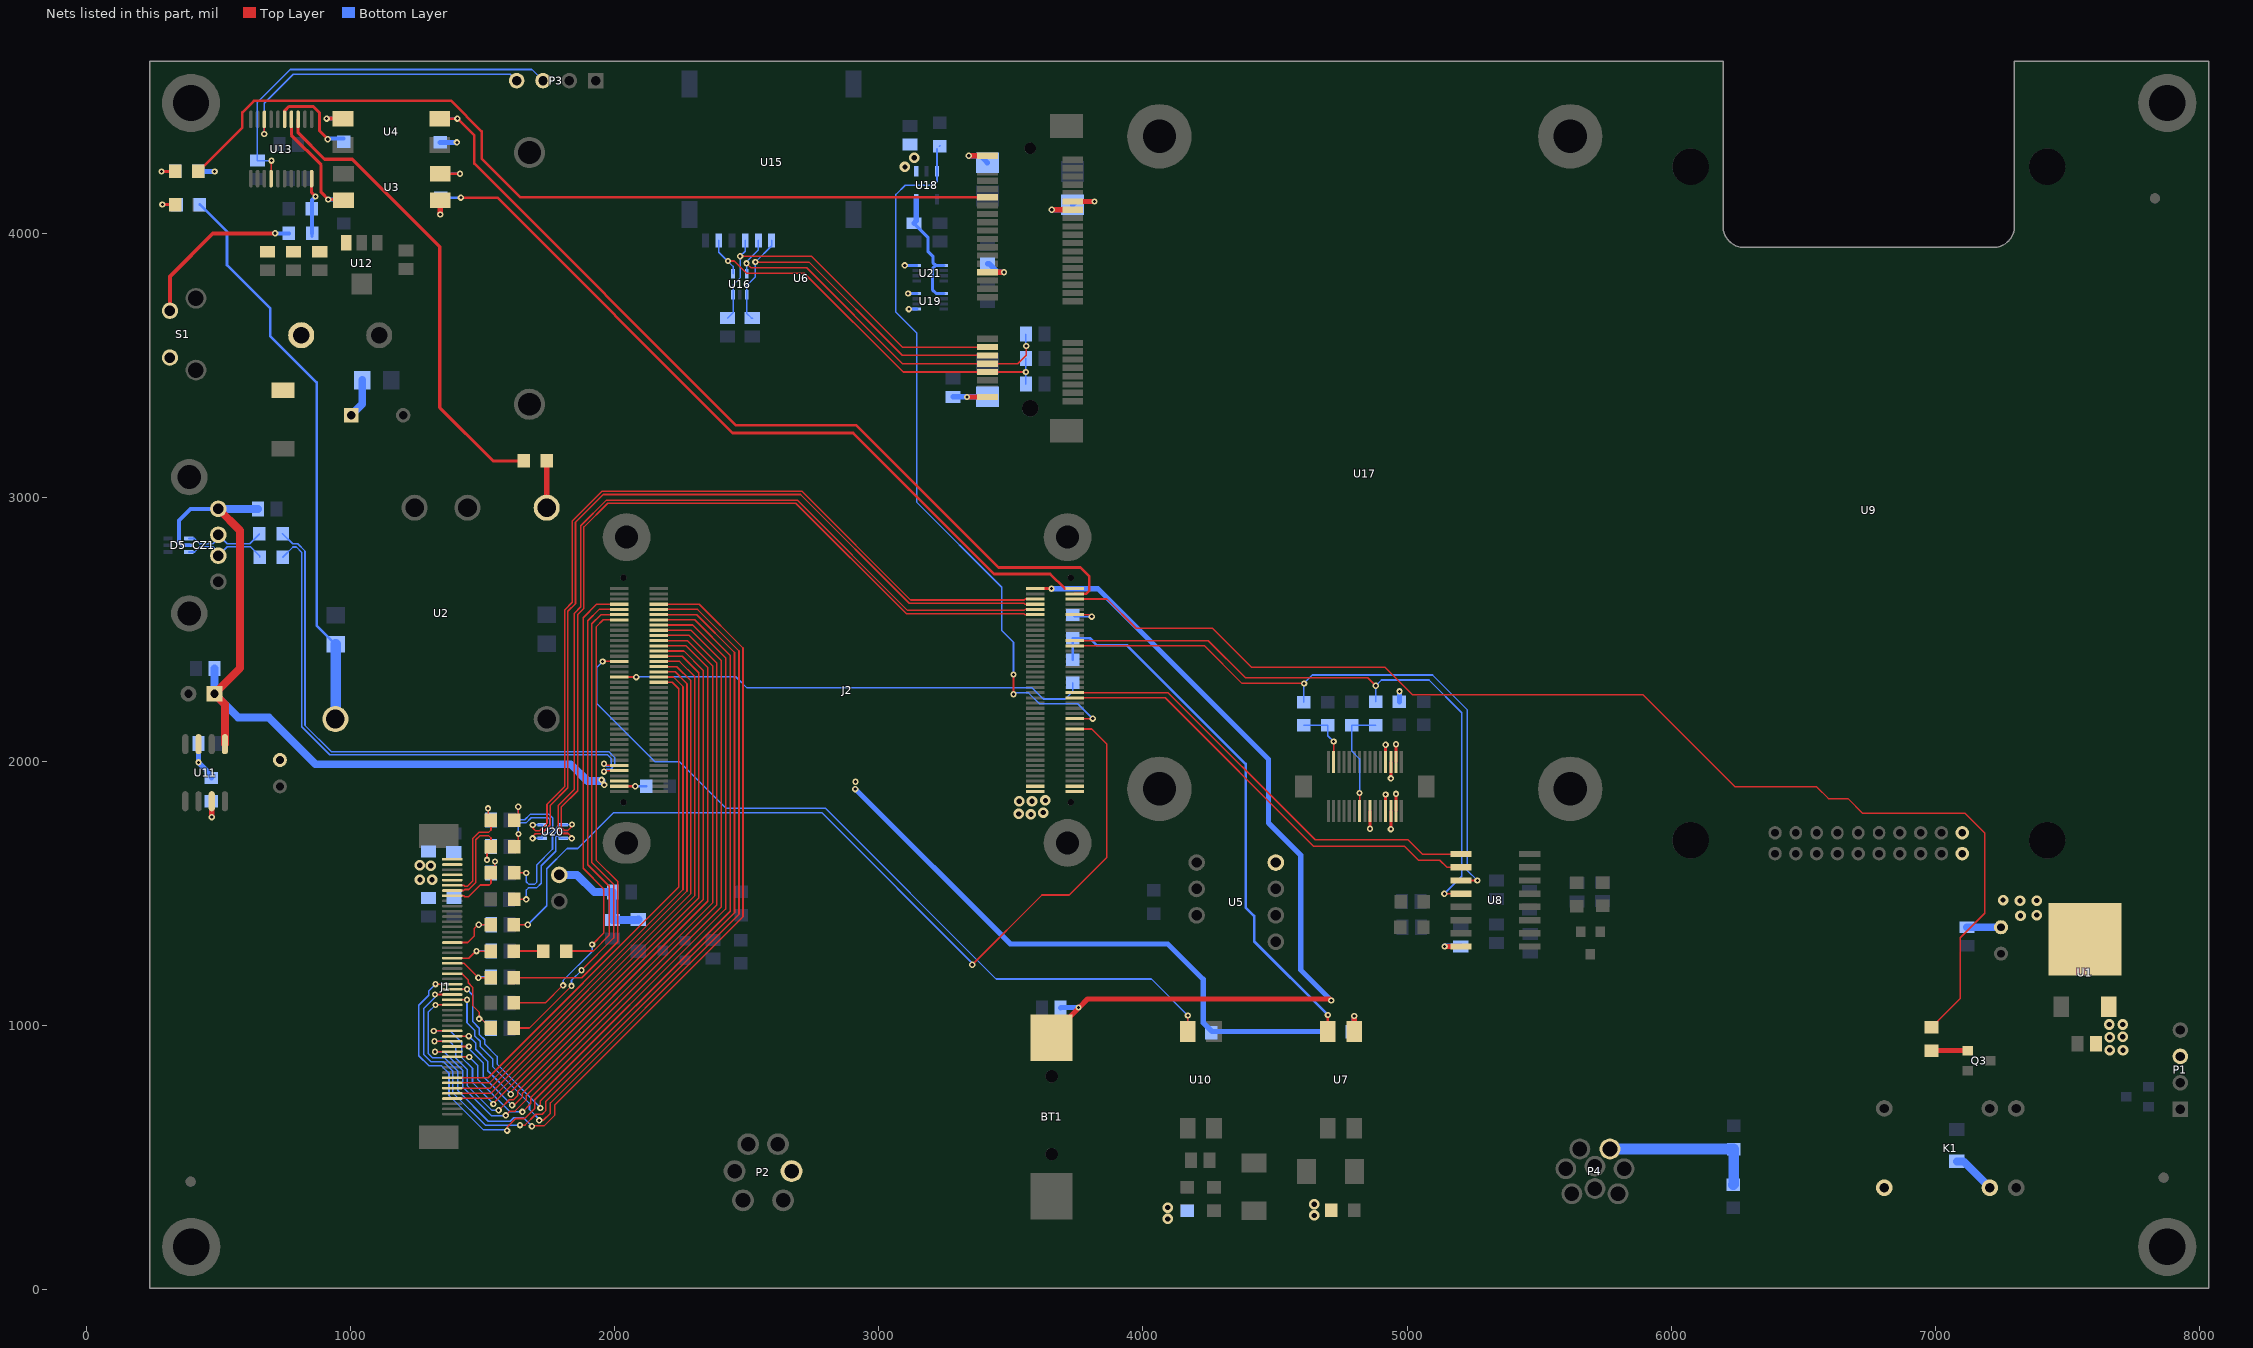
[diagram p0: the nets of this part, all layers, seen from the top]
# Altium PCB MISC82794.PcbDoc (part 4 of 5)
Units mil, origin at the board's own origin, x right, y up, seen from the top; angles counter-clockwise.
Board outline 7795.28 x 4645.67 mil, 4 copper layers (Top Layer, GND, POWER, Bottom Layer); 157 components, 133 nets, 768 pads, 456 vias.

## Via types
v1: diameter 24, hole 12, Top Layer to Bottom Layer, 258 vias
v2: diameter 40, hole 20, Top Layer to Bottom Layer, 197 vias
v3: diameter 30, hole 15, Top Layer to Bottom Layer, 1 vias

## Nets (pads, with @x,y where several pads share a name; then routed paths per layer and width w, separated by ;. In a path a pad name is that pad's centre, name@x,y a point inside that pad or via, vN(x,y) a via of type N, cw(c..) or ccw(c..) an arc to the next point about the centre after c; other vN are vias at no path point) (continued)
NetDD1_1: DD1.1 R1.1 | length 103
  Top Layer w10: v1(288.14,4108.86) DD1.1@337.14,4108.86
  Bottom Layer w10: v1(288.14,4108.86) R1.1@342.14,4108.86
NetDD2_1: DD2.1 R45.2 | length 102
  Top Layer w10: v1(285,4234) DD2.1@336,4234
  Bottom Layer w10: v1(285,4234) R45.2@336,4234
NetDD2_2: DD2.2 U6.42 | length 3342.4
  Top Layer w10: DD2.2@424,4234 591,4401 591,4457 635,4501 1382,4501 1497,4386 1497,4283 1643.79,4136.21 U6.42@3411.58,4136.21
NetJ2_A35: J2.A35 R37.2 | length 1796.2
  Top Layer w6: J2.A35@2017.8,2320.21 v1@2081.79,2320.21
  Bottom Layer w6: v1(2082,2320) 2083.53,2321.53 2459,2321.53 2501.53,2279 3581,2279 3623,2237 3671,2237 3706,2237 3734,2265 R37.2@3734,2298
NetJ2_B69: J2.B69 R36.2 | length 141.4
  Top Layer w6: J2.B69@3742.2,2556.43 3798.57,2556.43 v1(3806,2549)
  Bottom Layer w6: R36.2@3734,2555 3740,2549 v1(3806,2549)
NetL1_1: L1.1 R5.2 | length 110.2
  Top Layer w6: L1.1@1619,1282.6 1619.4,1283 R5.2@1729,1283
NetP4_3: P4.3 R39.1 R40.1 | length 601.8
  Bottom Layer w40: P4.3@5768.09,533.49 R40.1@6235.51,533.49 ; R39.1@6235,399 6236,400 R40.1@6236,533
NetQ3_1: Q3.1 R30.2 | length 122.7
  Top Layer w19.68: R30.2@7000,906 7121.9,906 Q3.1@7122.5,905.4
NetR8_1: R8.1 U2.6 | length 177
  Top Layer w6: R8.1@1744,3137 R8.1@1744,3138
  Top Layer w20: U2.6@1743,2961 R8.1@1743,3137
NetR8_2: R8.2 U13.13 | length 1776.4
  Top Layer w12: U13.13@801.98,4431.2 801.98,4380.02 902,4280 1006.92,4280 1338,3948.92 1338,3340 1540,3138 R8.2@1656,3138
NetR11_2: R11.2 U3.2 | length 148.8
  Top Layer w10: U3.2@1340.07,4225 v1(1415,4225)
  Bottom Layer w10: R11.2@1342,4223 1344,4225 v1(1415,4225)
NetR18_2: R18.2 U7.1 | length 122.1
  Top Layer w20: U7.1@4800,978.07 v1(4800,1037)
  Bottom Layer w20: R18.2@4790,978 4800,988 v1(4800,1037)
NetR24_1: R24.1 U11.3 | length 120.4
  Top Layer w20: v1(475,1790) U11.3@475,1849.97
  Bottom Layer w20: R24.1@474,1850 474,1791 v1(475,1790)
NetR29_1: R29.1 U4.1 | length 125.9
  Top Layer w15: v1(910,4434) U4.1@971.93,4434
  Bottom Layer w15: v1(910,4434) R29.1@974,4434
NetR29_2: R29.2 U13.15 | length 356.2
  Top Layer w12: U13.15@750.8,4431.2 750.8,4463.8 767,4480 859.77,4480 883,4456.77 883,4388 915,4356 v1(914,4356)
  Bottom Layer w15: v1@914,4358 R29.2@974,4358
NetR31_1: R31.1 S1.1 | length 699
  Top Layer w15: S1.1@316.79,3706.58 316.79,3836.79 480,4000 642,4000 ; 591,4000 642,4000 ; v1(715,4000) 642,4000
  Bottom Layer w15: v1(715,4000) R31.1@767,4000
NetR31_2: R31.2 R34.2 U13.10 | length 230.3
  Top Layer w12: U13.10@853.16,4206.79 853.16,4153.84 v1(868,4139)
  Bottom Layer w12: R31.2@854,3988 R31.2@854,4000
  Bottom Layer w15: R31.2@855,4000 855,4126 v1(868,4139)
NetR33_2: R33.2 U3.4 U13.14 | length 478.2
  Top Layer w12: U13.14@776.39,4431.2 776.39,4371.61 889,4259 889,4155 v1(916,4128) 970.93,4128 U3.4@973.93,4125
  Bottom Layer w15: v1(916,4128) R33.2@974,4128
NetR41_2: R41.2 R42.2 U17.3 | length 238.5
  Top Layer w6: U17.3@4721.89,1998.52 v1(4721.89,2075.89)
  Bottom Layer w6: R41.2@4609,2137 R42.2@4700,2137 4700,2097.78 v1(4721.89,2075.89)
NetR43_2: R43.2 R44.2 U17.14 | length 428.1
  Top Layer w6: v1(4820,1881) 4820.31,1880.69 U17.14@4820.31,1813.48
  Bottom Layer w6: v1(4820,1881) 4820,2010 4790,2040 R43.2@4790,2138 R44.2@4881,2138
OVER_LOAD: J2.A29 R21.2 U10.4 | length 3084.3
  Top Layer w6: v1(1954.73,2379.27) J2.A29@2017.8,2379.27 ; U10.4@4169,978.07 4170,979.07 v1(4170,1039)
  Bottom Layer w6: v1(1954.73,2379.27) 1933,2357.54 1933,2219.3 2152.3,2000 2245,2000 2421,1824 2797,1824 3444,1177 4032,1177 v1(4170,1039) R21.2@4170,974
POW_CTRL: J2.B75 R30.1 | length 4648.2
  Top Layer w6: J2.B75@3742.2,2615.49 3863.51,2615.49 3974.5,2504.5 4263.5,2504.5 4410,2358 4915,2358 5020,2253 5893,2253 6241,1905 6550,1905 6595,1860 6669,1860 6724,1805 7112,1805 7187,1730 7187,1426 7094,1333 7094,1103 R30.1@6985,994 ; R30.1@6983,977 R30.1@6983,994
POW_OFF: J2.B79 R11.1 | length 3019.3
  Top Layer w10: v1(1418,4135) 1433,4135 ; 1439,4135 1433,4135 ; J2.B79@3742.2,2654.86 3704.14,2654.86 3649,2710 3437,2710 2903,3244 2447,3244 1556,4135 1433,4135
  Bottom Layer w10: R11.1@1342,4135 v1(1418,4135)
POW_SW: J2.B77 R28.2 U4.4 | length 3418.3
  Top Layer w10: U4.4@1338.07,4434 v1(1405,4434) 1469,4370 1469,4264 2460,3273 2915,3273 3453,2735 3763,2735 3797,2701 3797,2647.17 3785,2635.17 J2.B77@3742.2,2635.17
  Bottom Layer w10: R28.2@1340,4432 1342,4434 v1(1405,4434)
POWER_OK: J2.B29 R46.1 U18.3 | length 2788.8
  Top Layer w6: v1(3510,2255) v1(3510,2330) ; J2.B29@3742.2,2162.73 v1(3809.73,2162.73)
  Bottom Layer w6: R46.1@3220.37,4320.37 U18.3@3220.37,4235.15 3220.37,4195.37 3207,4182 3100,4182 3065,4147 3065,3701 3143,3623 3143,2983 3466,2660 3466,2496 3510,2452 v1(3510,2330) ; R46.1@3230,4330 R46.1@3231.73,4331.73 ; v1(3510,2255) 3515,2260 3567,2260 3608,2219 3753.47,2219 v1(3809.73,2162.73)
PWM_LIGHT: C8.1 J1.17 R6.2 | length 236.9
  Top Layer w6: J1.17@1385.39,1315.17 1444.17,1315.17 1468,1339 1468,1367 1483.6,1382.6 v1(1486,1382.6) R6.2@1531,1382.6
  Bottom Layer w6: v1(1486,1382.6) C8.1@1533,1382.6
RESET: C34.2 P3.3 U13.4 | length 1490.6
  Top Layer w6: U13.4@699.61,4206.79 v1@699.61,4273.61
  Bottom Layer w6: v1(701,4275) C34.2@648,4275 648,4496 772,4620 1687,4620 P3.3@1729,4578
SWIM: P3.4 U13.18 | length 1181.7
  Top Layer w6: v1@674.02,4376.02 U13.18@674.02,4431.2
  Bottom Layer w6: v1(674,4376) 674,4492 784,4602 1605,4602 P3.4@1629,4578
TFT_B0: J1.29 J2.A8 | length 3374.5
  Top Layer w6: v1(1322.06,1078.94) J1.29@1385.39,1078.94 ; v1@1686,621 1733,621 1774,662 1774,701 2486,1413 2486,2430 2320.2,2595.8 J2.A8@2167.4,2595.8
  Bottom Layer w6: v1(1322.06,1078.94) 1294,1050.89 1294,896 1311,879 1356,879 1407,828 1407,754 1522,639 1605,639 1618,652 1655,652 v1(1687,620)
TFT_B1: J1.28 J2.A10 | length 3093.6
  Top Layer w6: J1.28@1385.39,1098.63 v1(1441.37,1098.63) ; v1(1715,642) 1730,642 1757,669 1757,708 2471,1422 2471,2419 2313.88,2576.12 J2.A10@2167.4,2576.12
  Bottom Layer w6: v1(1441.37,1098.63) 1441.37,1021 1441.37,1011.63 1471,982 1471,961 1491,941 1491,922 1538,875 1538,846 1678,706 1678,683 1715,646 v1(1715,642)
TFT_B2: J1.27 J2.A12 | length 3334.3
  Top Layer w6: v1(1320.32,1118.31) J1.27@1385.39,1118.31 ; v1(1642,624) 1661,624 1702,665 1726,665 1740,679 1740,713 1739.5,713.5 2454,1428 2454,2413 2310.57,2556.43 J2.A12@2167.4,2556.43
  Bottom Layer w6: v1(1320.32,1118.31) 1320.32,1108.31 1277,1065 1277,892 1305,864 1352,864 1388,828 1388,746 1510,624 1605,624 ; 1609,624 1605,624 ; v1(1642,624) 1605,624
TFT_B3: J1.26 J2.A14 | length 2957
  Top Layer w6: J1.26@1385.39,1138 v1(1441,1138) ; v1(1719,689) 1719,715 2438,1434 2438,2402 2303.25,2536.75 J2.A14@2167.4,2536.75
  Bottom Layer w6: v1(1441,1138) 1463,1116 1463,1016 1488,991 1488,967 1508,947 1508,931 1555,884 1555,855 1719,691 v1(1719,689)
TFT_B4: J1.25 J2.A16 | length 3315.6
  Top Layer w6: v1(1322.31,1157.69) J1.25@1385.39,1157.69 ; v1(1593,603) 1593,616 1626,649 1660,649 1698,687 1698,720 2420,1442 2420,2393 2295.94,2517.06 J2.A16@2167.4,2517.06
  Bottom Layer w6: v1(1322.31,1157.69) 1296.31,1131.69 1296.31,1115.31 1259,1078 1259,887 1298,848 1345,848 1373,820 1373,736 1502,607 v1@1593,607
TFT_BKLC: J2.B25 R6.1 | length 3486.5
  Top Layer w6: R6.1@1619,1382.6 v1(1671.4,1382.6) ; v1(3353.78,1230.78) 3618,1495 3721,1495 3863,1637 3863,2067 3806.64,2123.36 J2.B25@3742.2,2123.36
  Bottom Layer w6: v1(1671.4,1382.6) 1743,1454.2 1743,1594 1820,1671 1861,1671 1997,1807 2784,1807 3353.78,1237.22 v1(3353.78,1230.78)
TFT_G0: J1.39 J2.A18 | length 2683.5
  Top Layer w6: J1.39@1385.39,882.09 v1(1449.91,882.09) ; v1(1651,674) 1682,705 1682,728 2403,1449 2403,2384 2289.62,2497.38 J2.A18@2167.4,2497.38
  Bottom Layer w6: v1(1449.91,882.09) 1482,850 1482,797 1604,675 v1@1648,675
TFT_G1: J1.38 J2.A20 | length 2788.3
  Top Layer w6: v1(1320.22,901.78) J1.38@1385.39,901.78 ; v1(1588,661) 1604,677 1623,677 1665,719 1665,735 2387,1457 2387,2373 2282.31,2477.69 J2.A20@2167.4,2477.69
  Bottom Layer w6: v1(1320.22,901.78) 1354.22,901.78 1425,831 1425,768 1534,659 1586,659 v1(1588,661)
TFT_G2: J1.37 J2.A22 | length 2578.7
  Top Layer w6: J1.37@1385.39,921.46 v1(1448.46,921.46) ; v1(1612,699) 1619,699 1650,730 1650,744 2371,1465 2371,2363 2275.99,2458.01 J2.A22@2167.4,2458.01
  Bottom Layer w6: v1(1448.46,921.46) 1448.46,913.23 1502,859.7 1502,809 v1(1612,699)
TFT_G3: J1.36 J2.A24 | length 2714.5
  Top Layer w6: v1(1318.15,941.15) J1.36@1385.39,941.15 ; v1(1561,680) 1560,681 1560,687 1568,687 1601,720 1617,720 1634,737 1634,752 2353,1471 2353,2356 2270.68,2438.32 J2.A24@2167.4,2438.32
  Bottom Layer w6: v1(1318.15,941.15) 1374.85,941.15 1398,918 1398,879 1443,834 1443,772.3 1534.3,681 v1@1560,681
TFT_G4: J1.35 J2.A26 | length 2459.7
  Top Layer w6: J1.35@1385.39,960.83 v1(1448.17,960.83) ; v1@1610,740 1610,743 1608,741 v1(1607,741) 1607,749 2336,1478 2336,2345 2262.36,2418.64 J2.A26@2167.4,2418.64
  Bottom Layer w6: v1(1448.17,960.83) 1474,935 1474,911 1520,865 1520,830 v1@1608,742
TFT_G5: J1.34 J2.A28 | length 2616.5
  Top Layer w6: v1(1315.52,980.52) J1.34@1385.39,980.52 ; v1(1541,704) 1539,704 2319,1484 2319,2336 2256.05,2398.95 J2.A28@2167.4,2398.95
  Bottom Layer w6: v1(1315.52,980.52) 1378.32,980.52 1420.66,938.18 1420.66,880.34 1462,839 1462,785 1537,710 1537,702 1539,704 v1(1541,704)
TFT_HSYNC: J2.A7 R4.1 | length 1861.9
  Top Layer w6: R4.1@1619,1086.6 1737.6,1086.6 1805,1154 v1(1805,1153) ; v1@1915,1307 1959,1351 1959,1518 1881,1596 1881,2545 1931.8,2595.8 J2.A7@2017.8,2595.8
  Bottom Layer w6: v1(1805,1153) 1805,1171 1915,1281 v1(1915,1308)
TFT_R0: J1.47 J2.A30 | length 2225.6
  Top Layer w6: J1.47@1385.39,724.61 1385.78,725 1536,725 2304,1493 2304,2321 2245.73,2379.27 J2.A30@2167.4,2379.27
TFT_R1: J1.46 J2.A32 | length 2165.8
  Top Layer w6: J1.46@1385.39,744.3 1532.3,744.3 2289,1501 2289,2306 2235.42,2359.58 J2.A32@2167.4,2359.58
TFT_R2: J1.45 J2.A34 | length 2107.8
  Top Layer w6: J1.45@1385.39,763.98 1527.98,763.98 2274,1510 2274,2295 2229.1,2339.9 J2.A34@2167.4,2339.9
TFT_R3: J1.44 J2.A36 | length 2051.5
  Top Layer w6: J1.44@1385.39,783.67 1526.67,783.67 2259,1516 2259,2284 2222.79,2320.21 J2.A36@2167.4,2320.21
TFT_R4: J1.43 J2.A38 | length 1993.1
  Top Layer w6: J1.43@1385.39,803.35 1521.35,803.35 2243,1525 2243,2275.7 2218.17,2300.53 J2.A38@2167.4,2300.53
TFT_VCLK: J2.A9 R5.1 | length 1549.3
  Top Layer w6: R5.1@1817,1283 1919.7,1283 1980,1343.3 1980,1528 1898,1610 1898,2533 1941.12,2576.12 J2.A9@2017.8,2576.12
TFT_VDEN: J2.A13 R2.1 | length 1774.2
  Top Layer w6: R2.1@1619,1181.6 1875.3,1181.6 2012,1318.3 2012,1546 1930,1628 1930,2510 1956.75,2536.75 J2.A13@2017.8,2536.75
TFT_VSYNC: J2.A11 R3.1 | length 1872.9
  Top Layer w6: R3.1@1619,991.6 1677.6,991.6 v1(1837,1151) ; v1(1874.5,1210.5) 1996,1332 1996,1536 1914,1618 1914,2522 1948.43,2556.43 J2.A11@2017.8,2556.43
  Bottom Layer w6: v1(1837,1151) 1837,1172 1874.5,1209.5 v1(1874.5,1210.5)
TS_XM: J2.B74 R12.1 U20.4 | length 3621.6
  Top Layer w6: R12.1@1620,1778.6 1635,1793.6 v1(1635,1829) ; v1(1689.59,1709.41) 1689.59,1716.59 1700,1727 1722,1727 1756,1761 1756,1834 1823,1901 1823,2569.03 1852,2598.03 1852,2906 1957,3011 2704.03,3011 3115.38,2599.65 3549.89,2599.65 3553.74,2595.8 J2.B74@3592.6,2595.8
  Bottom Layer w6: v1(1635,1829) 1635,1788 1643,1780 1660,1780 1680,1800 1753,1800 1766,1787 1766,1741 1753,1728 1732,1728 1726.55,1722.55 U20.4@1726.55,1709.41 v1(1689.59,1709.41)
TS_XP: J2.B76 R14.1 U20.5 | length 3578.6
  Top Layer w6: R14.1@1620,1678.6 1636,1694.6 v1(1636,1726) ; v1(1690,1760) 1690,1749 1700,1739 1717,1739 1744,1766 1744,1838.97 1811,1905.97 1811,2574 1840,2603 1840,2910.97 1952.03,3023 2709,3023 3120.35,2611.65 3549.89,2611.65 3553.74,2615.49 J2.B76@3592.6,2615.49
  Bottom Layer w6: v1(1636,1726) 1636,1746 ; 1636,1750 1636,1746 ; v1@1691.41,1760.59 U20.5@1726.55,1760.59 1726.55,1746.45 1733,1740 1748,1740 1754,1746 1754,1782 1748,1788 1684.97,1788 1664.97,1768 1643,1768 1636,1761 1636,1746
TS_YM: J2.B70 R13.1 U20.1 | length 3580.6
  Top Layer w6: R13.1@1620,1578.6 v1(1665.6,1578.6) ; v1(1839,1762) 1840,1761 1840,1756 1824,1740 1809,1740 1798,1751 1798,1828.03 1860,1890.03 1860,2557.03 1884,2581.03 1884,2888 1974,2978 2686,2978 3103.72,2560.28 3549.89,2560.28 3553.74,2556.43 J2.B70@3592.6,2556.43
  Bottom Layer w6: v1(1665.6,1578.6) 1665.6,1545.4 1676,1535 1697,1535 1706,1544 1706,1610 1765,1669 1765,1720.03 1778.81,1733.84 1778.81,1748.81 1790.59,1760.59 U20.1@1805.45,1760.59 v1@1839.59,1760.59
TS_YP: J2.B72 R15.1 U20.3 | length 3599.6
  Top Layer w6: R15.1@1620,1478.6 v1(1665.6,1478.6) ; v1(1838,1709.41) 1838,1715 1825,1728 1804.03,1728 1786,1746.03 1786,1833 1848,1895 1848,2562 1872,2586 1872,2892.97 1969.03,2990 2690.97,2990 3108.69,2572.28 3549.89,2572.28 3553.74,2576.12 J2.B72@3592.6,2576.12
  Bottom Layer w6: v1(1665.6,1478.6) 1665.6,1513.6 1674,1522 1704,1522 1722,1540 1722,1606 1777,1661 1777,1715 1779.6,1717.6 1785.6,1717.6 1793.78,1709.41 U20.3@1805.45,1709.41 v1(1838,1709.41)
UART0_RXD: J2.B39 U8.9 | length 1714.9
  Top Layer w6: J2.B39@3742.2,2261.16 4094.84,2261.16 4652,1704 5003,1704 5057,1650 U8.9@5204,1650
UART0_TXD: J2.B37 U8.10 | length 1727.5
  Top Layer w6: J2.B37@3742.2,2241.47 4084.53,2241.47 4646,1680 4990,1680 5043,1627 5124,1627 5151,1600 U8.10@5204,1600
UART5_RXD: J2.B59 R44.1 U8.12 | length 2432.4
  Top Layer w6: J2.B59@3742.2,2458.01 4246.99,2458.01 4388,2317 4851,2317 v1(4881,2287) ; v1(5141,1500) U8.12@5204,1500
  Bottom Layer w6: R44.1@4881,2226 v1(4881,2287) 4903,2309 5083,2309 5207,2185 5207,1566 v1(5141,1500)
UART5_TXD: J2.B57 R41.1 U8.11 | length 2406.4
  Top Layer w6: J2.B57@3742.2,2438.32 4232.68,2438.32 4375,2296 v1@4599,2296 ; v1@4610,2287 v1(4610,2296) ; U8.11@5204,1550 v1(5266,1550)
  Bottom Layer w6: R41.1@4609,2225 4609,2296 4641,2328 5096,2328 5227,2197 5227,1589 v1(5266,1550)
USB0_H_N: CZ1.2 D5.4 R25.2 | length 327
  Bottom Layer w6: D5.4@388.45,2844.59 409.74,2844.59 429.33,2825 480,2825 500.12,2845.12 CZ1.2@500.12,2858.37 533.49,2825 619,2825 655,2861 R25.2@655,2863
USB0_H_P: CZ1.3 D5.6 R26.2 | length 330.2
  Bottom Layer w6: D5.6@388.45,2793.41 409.74,2793.41 429.33,2813 480,2813 500.12,2792.88 CZ1.3@500.12,2779.63 533.49,2813 622,2813 656,2779 R26.2@656,2774
USB0_ID: J2.A77 R27.2 | length 102.3
  Top Layer w10: J2.A77@2017.8,1906.83 v1(2078.17,1906.83)
  Bottom Layer w10: v1(2078.17,1906.83) 2078.35,1907 R27.2@2120,1907
USB0_N: J2.A71 R25.1 | length 2133.8
  Top Layer w6: v1(1960,1962) 1963.88,1965.88 J2.A71@2017.8,1965.88
  Bottom Layer w6: R25.1@743,2863 781.5,2824.5 800.5,2824.5 828,2797 828,2136.97 926.97,2038 1978,2038 2000,2016 2000,1986 1985,1971 1969,1971 v1(1960,1962)
USB0_P: J2.A69 R26.1 | length 2094.1
  Top Layer w6: v1(1960,1992) 1966.43,1985.57 J2.A69@2017.8,1985.57
  Bottom Layer w6: R26.1@744,2774 782.5,2812.5 795.53,2812.5 816,2792.03 816,2132 922,2026 1973.03,2026 1988,2011.03 1988,1990.97 1980.03,1983 1969,1983 v1(1960,1992)
USB0_VBUS_5V: C27.1 C28.1 C29.1 CZ1.1 D5.5 J2.A75 U11.5 | length 3121.5
  Top Layer w30: CZ1.1@500.12,2956.8 582,2874.91 582,2353.79 C27.1@485.21,2257 525,2217.21 U11.5@525,2066.03
  Bottom Layer w15: D5.5@388.45,2819 362,2819 351,2830 351,2913 394.8,2956.8 CZ1.1@500.12,2956.8
  Bottom Layer w30: C28.1@486,2353 486,2257.79 C27.1@485.21,2257 575.21,2167 691,2167 868,1990 1834,1990 1897,1927 v1@1950,1927 ; CZ1.1@500.12,2956.8 500.91,2956 C29.1@650,2956
  other v1: 1961,1912 1951,1931
USIM_CLK: C54.2 U6.12 U15.3 U16.1 | length 1371
  Top Layer w6: v1(2533,3891) 2736,3891 3089.21,3537.79 U6.12@3411.58,3537.79
  Bottom Layer w6: C54.2@2523,3679 2518,3679 2499.59,3697.41 U16.1@2499.59,3767.55 2499.59,3801.59 2533,3835 v1(2533,3891) 2594.39,3952.39 U15.3@2594.39,3973.23
USIM_DATA: C52.1 U6.10 U15.7 U16.5 | length 1453.2
  Top Layer w6: v1(2499.59,3886) 2516.59,3869 2727,3869 3089.71,3506.29 3359,3506.29 U6.10@3411.58,3506.29 3526.29,3506.29 3558,3538 v1(3558,3573)
  Bottom Layer w6: U16.5@2499.59,3846.45 2499.59,3892.59 2544.39,3937.39 U15.7@2544.39,3973.23 ; v1@3557,3574 C52.1@3557,3618
USIM_PWR: C50.1 C51.1 U6.8 U15.1 U16.4 | length 1548
  Top Layer w6: v1(2429,3895) 2453,3895 2499,3849 2718,3849 3092.2,3474.8 U6.8@3411.58,3474.8 v1@3556.8,3474.8
  Bottom Layer w6: U15.1@2394.39,3973.23 2394.39,3928.61 2448.41,3874.59 U16.4@2448.41,3846.45 ; C50.1@3557,3429 v1(3557,3475) C51.1@3557,3526
USIM_RST: C55.2 U6.14 U15.2 U16.3 | length 1400.7
  Top Layer w6: v1(2475,3913) 2745,3913 3088.72,3569.28 U6.14@3411.58,3569.28
  Bottom Layer w6: C55.2@2428,3679 2448.41,3699.41 U16.3@2448.41,3767.55 2448.41,3804.41 2475,3831 v1(2475,3913) 2494.39,3932.39 U15.2@2494.39,3973.23
VCLK: C9.1 J1.20 L1.2 | length 212.7
  Top Layer w6: J1.20@1385.39,1256.11 1448.11,1256.11 1474.6,1282.6 v1(1477,1282.6) L1.2@1531,1282.6
  Bottom Layer w6: v1(1477,1282.6) 1477.4,1283 C9.1@1533,1283
VDD_1.8: C58.2 U18.5 U19.1 U21.1 | length 464.9
  Bottom Layer w12: C58.2@3133,4038 3186,3985 3186,3932 3205,3913 3205,3889.06 3215.53,3878.53 ; U21.1@3246.18,3878.53 3215.53,3878.53 ; U19.1@3246.45,3772 3217,3772 3204,3785 3204,3867 3215.53,3878.53
  Bottom Layer w20: C58.2@3133,4038 3141.63,4046.63 U18.5@3141.63,4128.85
VDD_3.3: C1.1 C5.1 C19.2 C20.2 C39.1 C47.1 C48.1 C49.1 C56.1 C57.1 C59.2 J1.4 J1.5 R18.1 R21.1 R28.1 R45.1 R49.2 U1.2 U3.1 U5.4 U6.2 U6.24 U6.39 U6.41 U6.52 U8.16 U9.2 U17.18 U17.23 U17.24 U17.25 U17.26 U17.27 U17.28 U18.1 U19.5 U19.8 U21.8 | length 4112.7
  Top Layer w11: v1(4859.69,1745.69) U17.18@4859.69,1813.48 ; U17.24@4918.74,1813.48 v1(4918.74,1875.74) ; U17.23@4918.74,1998.52 v1(4918.74,2063.74) ; v1(4938.43,1744.43) U17.26@4938.43,1813.48 ; v1(4938.43,1936.57) U17.25@4938.43,1998.52 ; U17.28@4958.11,1813.48 v1(4958.11,1877.89) ; U17.27@4958.11,1998.52 v1(4958.11,2065.89)
  Top Layer w20: v1(1340.07,4071.07) U3.1@1340.07,4125 ; v1(3333.69,3380.31) U6.2@3411.58,3380.31 ; v1(3340.69,4293.69) U6.52@3411.58,4293.69 ; U6.24@3411.58,3852.75 v1(3474.25,3852.75) ; v1(3655.03,4088.97) U6.39@3734.42,4088.97 ; U6.41@3734.42,4120.46 v1(3816.46,4120.46) ; v1(5142,1300) U8.16@5204,1300
  Bottom Layer w11: v1(3098.47,3878.53) U21.8@3143.82,3878.53 ; v1(3111,3772) U19.8@3144.08,3772 ; v1(3113.94,3712.94) U19.5@3144.08,3712.94
  Bottom Layer w20: R45.1@424,4234 v1(486,4234) ; R28.1@1340,4344 v1(1403,4344) ; v1@2911,1897 3498,1310 4094,1310 4228,1176 4228,1012 4262,978 R18.1@4702,978 ; C57.1@3281,3381 3333,3381 v1(3333.69,3380.31) 3334.39,3381.01 C48.1@3412,3381.01 ; v1(3340.69,4293.69) 3384.3,4293.69 C47.1@3411,4266.99 ; C56.1@3412,3885 3417,3885 3449.25,3852.75 v1(3474.25,3852.75) ; v1(3655.03,4088.97) C49.1@3714.96,4088.97 ; C49.1@3734,4108.01 3746.46,4120.46 v1(3816.46,4120.46) ; R49.2@4971,2227 v1(4971,2266) ; v1(5142,1300) 5143,1301 C39.1@5203,1301
  Bottom Layer w30: C5.1@7120,1373 C1.1@7248,1373
  other v1: 2911,1896 2912,1924
  other v2: 7322,1417 7383,1419 7320,1473 7383,1474 7256,1476 1263,1553 1309,1553 3099,4251 3134,4286
VDD_5V: BZ1.1 C2.1 C3.1 C4.2 C6.1 C7.2 C21.1 C22.2 C26.2 D1.2 D10.2 J1.1 J1.2 J2.B1 J2.B2 J2.B3 J2.B4 K1.4 P1.3 R1.2 R24.2 U1.3 U2.3 U9.1 U11.7 | length 2908.8
  Bottom Layer w10: R1.2@430.14,4108.86 533,4006 533,3957 533,3951 533,3879 697,3715 697,3610 872,3435 872,2515.88 C4.2@944,2443.88
  Bottom Layer w20: C26.2@425,2069 v1(425,1997) 474,1948 R24.2@474,1938
  Bottom Layer w30: BZ1.1@1791,1571 1858,1571 1923,1506 C3.1@1993,1506 ; C3.1@1992,1505 C7.2@1992,1401 2089,1401 D1.2@2090,1402 ; D10.2@7081,487 7106,487 K1.4@7206,387
  Bottom Layer w40: U2.3@944,2162 C4.2@944,2443.88
  other v2: 7710,907 7660,908 7660,957 7709,959 7658,1005 7709,1005 1304,1606 1262,1608 3576,1800 3530,1802 3623,1807 3532,1850 3580,1850 3631,1853
VDD_12V: C18.1 C23.2 C30.1 C31.1 C36.1 K1.1 L2.1 P2.2 R16.2 R17.2 R22.2 S1.2 U12.3 | length 150.5
  Bottom Layer w30: C36.1@1002.57,3311 1044.88,3353.31 C23.2@1044.88,3444
  other v2: 4094,269 4649,282 4094,312 4648,324
VDD_BAT: BT1.1 C24.1 J2.B80 | length 3359.2
  Top Layer w11: J2.B80@3592.6,2654.86 v1(3653.86,2654.86)
  Top Layer w20: BT1.1@3654,955 3654,965 v1@3757,1068 ; v1(3756,1069) v1@3757,1068 ; v1(4713,1096) 4708,1101 3790,1101 v1@3757,1068
  Bottom Layer w20: v1(3653.86,2654.86) 3829.14,2654.86 4475,2009 4475,1768 4597,1646 4597,1212 v1(4713,1096) ; C24.1@3688,1067 3690,1069 v1(3756,1069)
VDEN: C12.1 J1.21 R2.2 | length 217.2
  Top Layer w6: J1.21@1385.39,1236.43 1429.57,1236.43 v1(1484.4,1181.6) R2.2@1531,1181.6
  Bottom Layer w6: v1(1484.4,1181.6) 1487.4,1184.6 C12.1@1532,1184.6
VSYNC: C11.1 J1.23 R3.2 | length 342.9
  Top Layer w6: J1.23@1385.39,1197.06 1421.94,1197.06 1446,1173 1446,1162.7 1462.37,1146.33 1462.37,1076.63 1487,1052 v1(1487,1026) ; v1@1496.6,1026 R3.2@1531,991.6
  Bottom Layer w6: v1(1487,1026) 1496.6,1026 C11.1@1532,990.6
WH_SPEED: R36.1 R37.1 U7.2 | length 2074.9
  Top Layer w10: U7.2@4700,978.07 v1(4700,1041)
  Bottom Layer w10: R37.1@3734,2386 R36.1@3734,2467 3800,2467 3827,2440 3940,2440 4389,1991 4389,1448 4421,1416 4421,1320 v1(4700,1041)
XM: C17.1 J1.6 R12.2 | length 466.3
  Top Layer w6: J1.6@1385.39,1531.7 1428.74,1531.7 1432.58,1527.86 1442.89,1527.86 1462.83,1547.8 1462.83,1708.8 1486.03,1732 1523,1732 1532,1741 R12.2@1532,1778.6 1521,1789.6 v1(1521,1823)
  Bottom Layer w6: v1(1521,1823) 1521,1789.6 C17.1@1532,1778.6
XP: C15.1 J1.7 R14.2 | length 476.8
  Top Layer w6: J1.7@1385.39,1512.02 1428.74,1512.02 1432.58,1515.86 1447.86,1515.86 1474.83,1542.83 1474.83,1703.83 1491,1720 1523,1720 1532,1711 R14.2@1532,1678.6 1517,1663.6 v1(1517,1628)
  Bottom Layer w6: v1(1517,1628) 1517,1663.6 C15.1@1532,1678.6
YM: C16.1 J1.8 R13.2 | length 308.9
  Top Layer w6: J1.8@1385.39,1492.33 1428.74,1492.33 1432.58,1488.49 1447,1488.49 1491.51,1533 1526,1533 1532,1539 R13.2@1532,1578.6 1547,1593.6 v1(1547,1622)
  Bottom Layer w6: C16.1@1532,1577.6 1547,1592.6 v1(1547,1622)